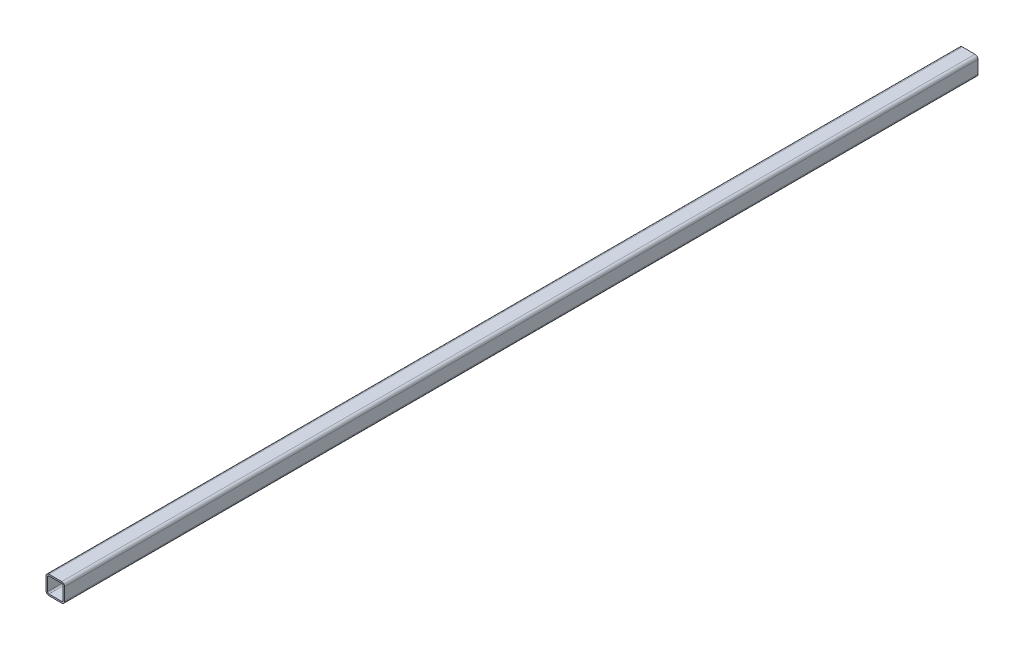
from build123d import *

# Parameters (mm, degrees)
BOSS_EXTRUDE1_DEPTH = 1224


with BuildPart() as part:
    # Sketch1 → Boss-Extrude1 (new body)
    with BuildSketch(Plane.XY):
        with BuildLine():
            Line((-8.5, -12.5), (8.5, -12.5))
            ThreePointArc((8.5, -12.5), (11.328427125, -11.328427125), (12.5, -8.5))
            Line((12.5, -8.5), (12.5, 8.5))
            ThreePointArc((12.5, 8.5), (11.328427125, 11.328427125), (8.5, 12.5))
            Line((8.5, 12.5), (-8.5, 12.5))
            ThreePointArc((-8.5, 12.5), (-11.328427125, 11.328427125), (-12.5, 8.5))
            Line((-12.5, 8.5), (-12.5, -8.5))
            ThreePointArc((-12.5, -8.5), (-11.328427125, -11.328427125), (-8.5, -12.5))
        make_face()
        with BuildLine():
            Line((-8.5, -10.5), (8.5, -10.5))
            ThreePointArc((8.5, -10.5), (9.914213562, -9.914213562), (10.5, -8.5))
            Line((10.5, -8.5), (10.5, 8.5))
            ThreePointArc((10.5, 8.5), (9.914213562, 9.914213562), (8.5, 10.5))
            Line((8.5, 10.5), (-8.5, 10.5))
            ThreePointArc((-8.5, 10.5), (-9.914213562, 9.914213562), (-10.5, 8.5))
            Line((-10.5, 8.5), (-10.5, -8.5))
            ThreePointArc((-10.5, -8.5), (-9.914213562, -9.914213562), (-8.5, -10.5))
        make_face(mode=Mode.SUBTRACT)
    extrude(amount=BOSS_EXTRUDE1_DEPTH)


solid = part.part
